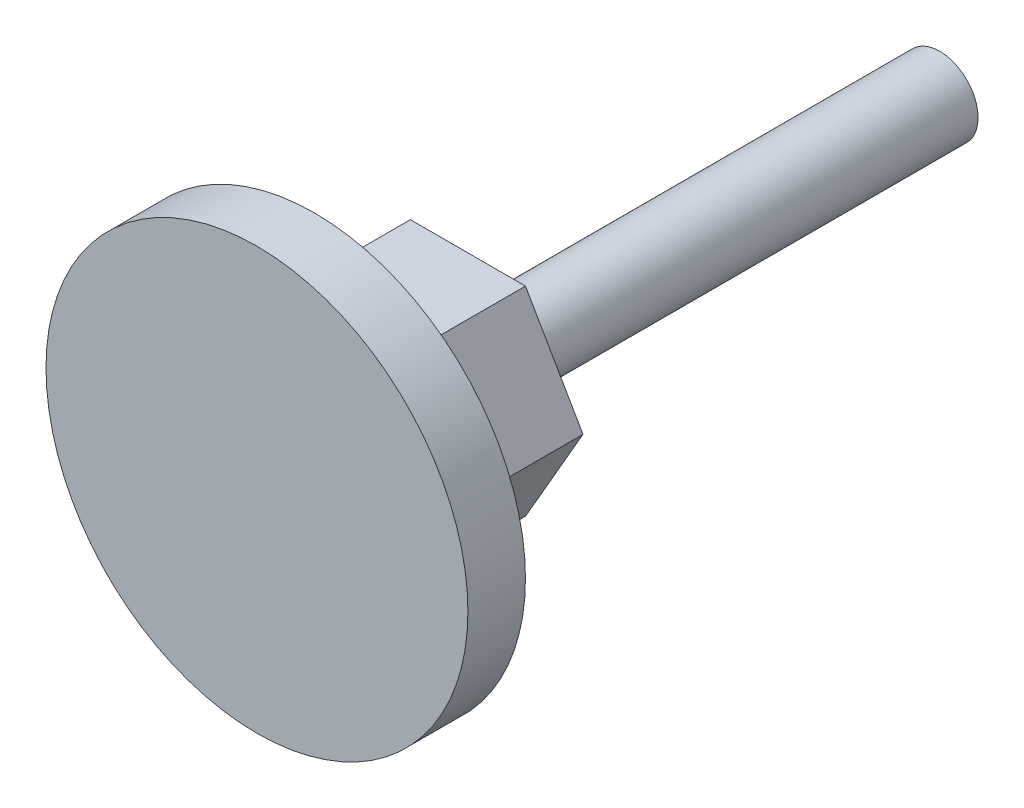
SolidWorks part; units mm, degrees
ref_plane "前视基准面" through (0, 0, 0) normal (0, 0, 1) x (1, 0, 0)
ref_plane "上视基准面" through (0, 0, 0) normal (0, 1, 0) x (1, 0, 0)
ref_plane "右视基准面" through (0, 0, 0) normal (1, 0, 0) x (0, 0, -1)
sketch "草图1" plane through (0, 0, 0) normal (0, 1, 0) x (1, 0, 0)
  line L0 (0, 40) -> (0, -123) construction
  line L1 (0, 40) -> (-10, 40)
  line L2 (-10, 40) -> (-10, -108)
  line L3 (-10, -108) -> (-25, -108)
  line L4 (-55, -123) -> (0, -123)
  line L6 (0, 40) -> (0, -123)
  line L7 (-25, -108) -> (-55, -123)
  dimension "D1" = 10
  dimension "D2" = 55
  dimension "D3" = 15
  dimension "D5" = 40
  dimension "D6" = 148
  dimension "D7" = 15
revolve "旋转1" add sketch "草图1" angle 360 about L0
cosmetic thread "装饰螺纹线2"
sketch "草图2" plane through (0, 0, 123) normal (0, 0, 1) x (1, 0, 0)
  circle A1 centre (0, 0) radius 55
  circle A2 centre (0, 0) radius 55
  dimension "D1" = 0
extrude "凸台-拉伸1" add sketch "草图2" along normal blind 15
sketch "草图3" plane through (0, 0, 108) normal (0, 0, -1) x (-1, 0, 0)
  line L1 (15, 25.9808) -> (-15, 25.9808)
  line L2 (-15, 25.9808) -> (-30, 0)
  line L3 (-30, 0) -> (-15, -25.9808)
  line L4 (-15, -25.9808) -> (15, -25.9808)
  line L5 (15, -25.9808) -> (30, 0)
  line L6 (30, 0) -> (15, 25.9808)
  circle A0 centre (0, 0) radius 25.9808 construction
extrude "凸台-拉伸2" add sketch "草图3" along normal blind 25
ref_plane "基准面1" through (0, 0, 95.5) normal (0, 0, -1) x (-1, 0, 0)
sketch "草图4" plane through (0, 0, 0) normal (0, 1, 0) x (1, 0, 0)
  line L0 (-30, -37.3068) -> (-30, -83)
  line L2 (-30, -83) -> (-19.7494, -35)
  arc A0 (-19.7494, -35) -> (-30, -37.3068) centre (30, -280) ccw
  dimension "D1" = 500
  dimension "D2" = 280
  dimension "D3" = 30
revolve "切除-旋转3" [suppressed] cut sketch "草图4" angle 360
mirror "镜向1" [suppressed] about plane through (0, 0, 95.5) normal (0, 0, -1)
